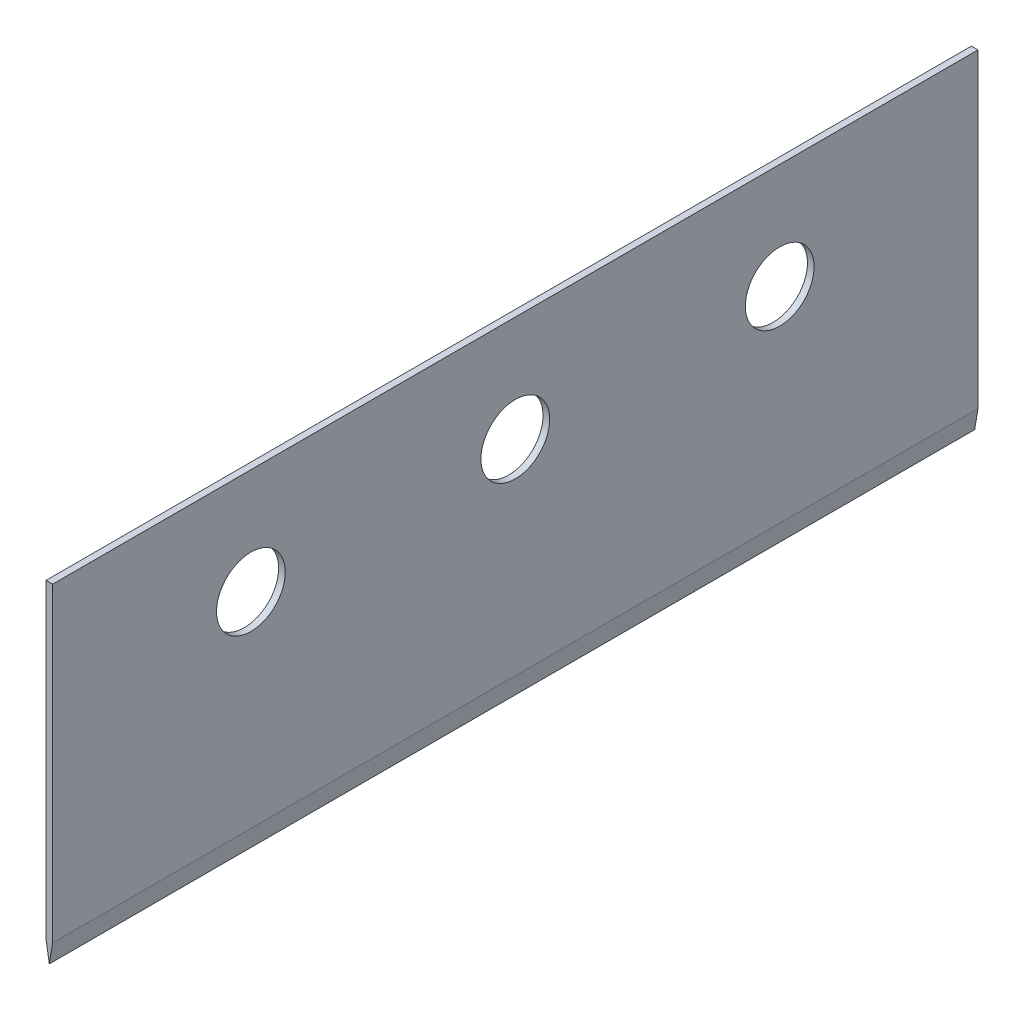
from build123d import *

# Parameters (mm, degrees)
SKETCH_1_W                  = 70
SKETCH_1_H                  = 25
EXTRUDE_1_DEPTH             = 0.5
CUT_EXTRUDE_1_DEPTH         = 72.109071151
HOLE_WIZARD_5_2_5_2_1_D     = 5.2
HOLE_WIZARD_5_2_5_2_1_DEPTH = 19.75
HOLE_WIZARD_5_2_5_2_1_TIP   = 1.562237609


with BuildPart() as part:
    # 草图1 → 凸台-拉伸1 (new body)
    with BuildSketch(Plane(origin=(0, 0, 0), x_dir=(0, 0, -1), z_dir=(1, 0, 0))):
        Rectangle(SKETCH_1_W, SKETCH_1_H)
    extrude(amount=EXTRUDE_1_DEPTH)

    # 草图2 → 切除-拉伸1 (cut, through all)
    with BuildSketch(Plane.XY.offset(35)):
        Polygon((0.25, -12.5), (0, -11), (-1.209013091, -11.201502182), (-0.510365148, -13.117899248), (1.363353431, -13.117899248), (1.198992152, -10.8497136), (0.5, -11), align=None)
    extrude(amount=-CUT_EXTRUDE_1_DEPTH, mode=Mode.SUBTRACT)

    # Ø5.2 (5.2) 直径孔1
    with Locations(Plane.ZY):
        with Locations((-20, 4.5), (0, 4.5), (20, 4.5)):
            Hole(HOLE_WIZARD_5_2_5_2_1_D / 2, depth=HOLE_WIZARD_5_2_5_2_1_DEPTH)
            with Locations((0, 0, -(HOLE_WIZARD_5_2_5_2_1_DEPTH + HOLE_WIZARD_5_2_5_2_1_TIP / 2))):  # 118° drill point
                Cone(0, HOLE_WIZARD_5_2_5_2_1_D / 2, HOLE_WIZARD_5_2_5_2_1_TIP, mode=Mode.SUBTRACT)


solid = part.part
